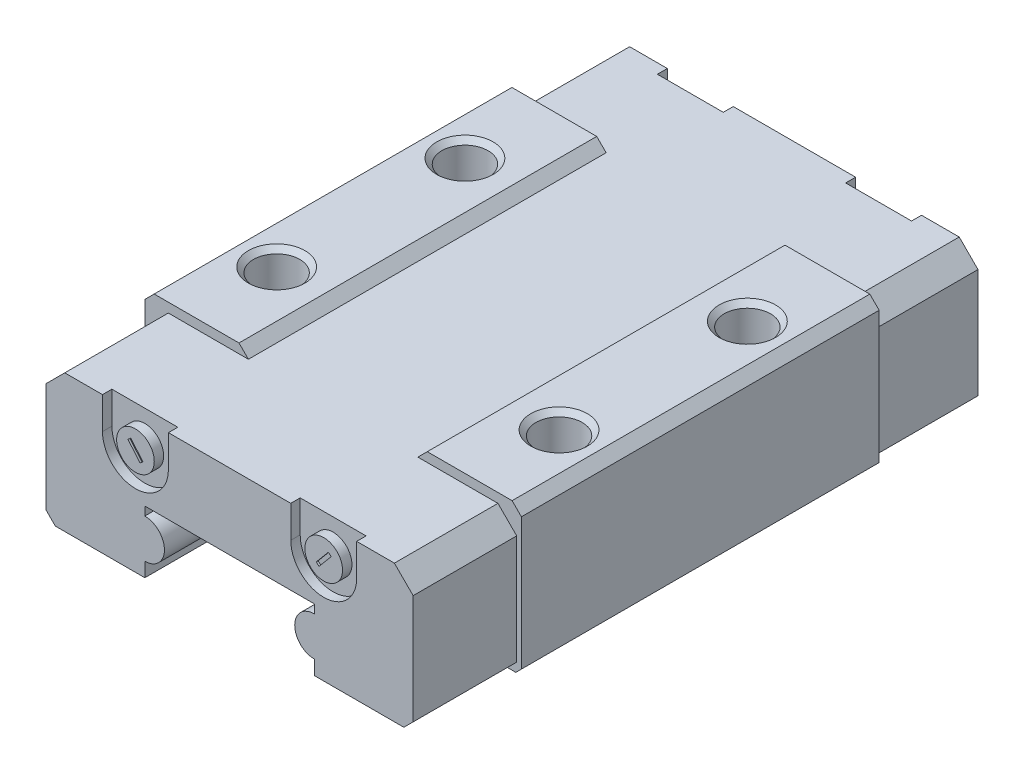
from build123d import *

# Parameters (mm, degrees)
BOSS_EXTRUDE1_DEPTH      = 9.5
BOSS_EXTRUDE1_DEPTH_BACK = 9.5
BOSS_EXTRUDE2_DEPTH      = 5.5
BOSS_EXTRUDE3_START      = -5.5
BOSS_EXTRUDE3_DEPTH      = 5.5
SKETCH4_R                = 1
CUT_EXTRUDE1_DEPTH       = 0.53
CUT_EXTRUDE2_START       = -0.5
SKETCH5_R                = 1
CUT_EXTRUDE2_DEPTH       = 0.5
LPATTERN1_COUNT          = 2
LPATTERN1_PITCH          = 10
LPATTERN1_COUNT_DIR2     = 2
LPATTERN1_PITCH_DIR2     = 15
CUT_EXTRUDE3_DEPTH       = 0.1
CUT_EXTRUDE4_DEPTH       = 0.1
CUT_EXTRUDE5_DEPTH       = 0.1
CUT_EXTRUDE6_DEPTH       = 0.1


with BuildPart() as part:
    # Sketch1 → Boss-Extrude1 (new, two sides: drawn at the far end of the back side and taken through both)
    with BuildSketch(Plane.XY.offset(-BOSS_EXTRUDE1_DEPTH_BACK)):
        with BuildLine():
            Line((-10, 7.305025253), (-10, 0.296984848))
            Line((-10, 0.296984848), (-9.703015152, 0))
            Line((-9.703015152, 0), (-4.5, 0))
            Line((-4.5, 0), (-4.5, 0.76))
            ThreePointArc((-4.5, 0.76), (-3.46, 1.8), (-4.5, 2.84))
            Line((-4.5, 2.84), (-4.5, 3.3))
            Line((-4.5, 3.3), (4.5, 3.3))
            Line((4.5, 3.3), (4.5, 2.84))
            ThreePointArc((4.5, 2.84), (3.46, 1.8), (4.5, 0.76))
            Line((4.5, 0.76), (4.5, 0))
            Line((4.5, 0), (9.703015152, 0))
            Line((9.703015152, 0), (10, 0.296984848))
            Line((10, 0.296984848), (10, 7.305025253))
            Line((10, 7.305025253), (9.505025253, 7.8))
            Line((9.505025253, 7.8), (5, 7.8))
            Line((5, 7.8), (4.5, 7.3))
            Line((4.5, 7.3), (-4.5, 7.3))
            Line((-4.5, 7.3), (-5, 7.8))
            Line((-5, 7.8), (-9.505025253, 7.8))
            Line((-9.505025253, 7.8), (-10, 7.305025253))
        make_face()
    extrude(amount=BOSS_EXTRUDE1_DEPTH + BOSS_EXTRUDE1_DEPTH_BACK)

    # Sketch2 → Boss-Extrude2 (add)
    with BuildSketch(Plane.XY.offset(9.5)):
        with BuildLine():
            Line((-9.75, 6.302979439), (-9.75, 0.494974747))
            Line((-9.75, 0.494974747), (-9.255025253, 0))
            Line((-9.255025253, 0), (-4.5, 0))
            Line((-4.5, 0), (-4.5, 0.76))
            ThreePointArc((-4.5, 0.76), (-3.46, 1.8), (-4.5, 2.84))
            Line((-4.5, 2.84), (-4.5, 3.3))
            Line((-4.5, 3.3), (4.5, 3.3))
            Line((4.5, 3.3), (4.5, 2.84))
            ThreePointArc((4.5, 2.84), (3.46, 1.8), (4.5, 0.76))
            Line((4.5, 0.76), (4.5, 0))
            Line((4.5, 0), (9.255025253, 0))
            Line((9.255025253, 0), (9.75, 0.494974747))
            Line((9.75, 0.494974747), (9.75, 6.302979439))
            Line((9.75, 6.302979439), (8.752979439, 7.3))
            Line((8.752979439, 7.3), (-8.752979439, 7.3))
            Line((-8.752979439, 7.3), (-9.75, 6.302979439))
        make_face()
    extrude(amount=BOSS_EXTRUDE2_DEPTH)

    # Sketch3 → Boss-Extrude3 (add)
    with BuildSketch(Plane.XY.offset(-9.5).offset(BOSS_EXTRUDE3_START)):
        with BuildLine():
            Line((-9.75, 6.302979439), (-9.75, 0.494974747))
            Line((-9.75, 0.494974747), (-9.255025253, 0))
            Line((-9.255025253, 0), (-4.5, 0))
            Line((-4.5, 0), (-4.5, 0.76))
            ThreePointArc((-4.5, 0.76), (-3.46, 1.8), (-4.5, 2.84))
            Line((-4.5, 2.84), (-4.5, 3.3))
            Line((-4.5, 3.3), (4.5, 3.3))
            Line((4.5, 3.3), (4.5, 2.84))
            ThreePointArc((4.5, 2.84), (3.46, 1.8), (4.5, 0.76))
            Line((4.5, 0.76), (4.5, 0))
            Line((4.5, 0), (9.255025253, 0))
            Line((9.255025253, 0), (9.75, 0.494974747))
            Line((9.75, 0.494974747), (9.75, 6.302979439))
            Line((9.75, 6.302979439), (8.752979439, 7.3))
            Line((8.752979439, 7.3), (-8.752979439, 7.3))
            Line((-8.752979439, 7.3), (-9.75, 6.302979439))
        make_face()
    extrude(amount=BOSS_EXTRUDE3_DEPTH)

    # Sketch4 → Cut-Extrude1 (cut)
    with BuildSketch(Plane.XY.offset(-15)):
        with BuildLine():
            Line((-6.75, 20), (-6.75, 5.6))
            ThreePointArc((-6.75, 5.6), (-5, 3.85), (-3.25, 5.6))
            Line((-3.25, 5.6), (-3.25, 18.82500207))
            Line((-3.25, 18.82500207), (3.25, 18.82500207))
            Line((3.25, 18.82500207), (3.25, 5.6))
            ThreePointArc((3.25, 5.6), (5, 3.85), (6.75, 5.6))
            Line((6.75, 5.6), (6.75, 20))
            Line((6.75, 20), (-6.75, 20))
        make_face()
        with Locations((5, 5.6)):
            Circle(SKETCH4_R, mode=Mode.SUBTRACT)
        with Locations((-5, 5.6)):
            Circle(SKETCH4_R, mode=Mode.SUBTRACT)
    extrude(amount=CUT_EXTRUDE1_DEPTH, mode=Mode.SUBTRACT)

    # Sketch5 → Cut-Extrude2 (cut)
    with BuildSketch(Plane.XY.offset(15).offset(CUT_EXTRUDE2_START)):
        with BuildLine():
            Line((-6.75, 20), (-6.75, 5.6))
            ThreePointArc((-6.75, 5.6), (-5, 3.85), (-3.25, 5.6))
            Line((-3.25, 5.6), (-3.25, 18.82500207))
            Line((-3.25, 18.82500207), (3.25, 18.82500207))
            Line((3.25, 18.82500207), (3.25, 5.6))
            ThreePointArc((3.25, 5.6), (5, 3.85), (6.75, 5.6))
            Line((6.75, 5.6), (6.75, 20))
            Line((6.75, 20), (-6.75, 20))
        make_face()
        with Locations((5, 5.6)):
            Circle(SKETCH5_R, mode=Mode.SUBTRACT)
        with Locations((-5, 5.6)):
            Circle(SKETCH5_R, mode=Mode.SUBTRACT)
    extrude(amount=CUT_EXTRUDE2_DEPTH, mode=Mode.SUBTRACT)

    # Sketch6 → Cut-Revolve1 (revolve, cut)
    with BuildSketch(Plane(origin=(7.5, 0, 0), x_dir=(0, 0, -1), z_dir=(1, 0, 0)), mode=Mode.PRIVATE) as cut_revolve1_sk:
        Polygon((-5, 7.8), (-3.5, 7.8), (-3.7705, 7.5295), (-3.7705, 4.009852156), (-5, 3.3), align=None)
    cut_revolve1 = revolve(cut_revolve1_sk.sketch.rotate(Axis((7.5, 3.3, 5), (0, 1, 0)), 180), axis=Axis((7.5, 3.3, 5), (0, 1, 0)), mode=Mode.SUBTRACT)

    # LPattern1: Cut-Revolve1 2 × 2
    with Locations(*[(-j * LPATTERN1_PITCH_DIR2, 0, -i * LPATTERN1_PITCH) for i in range(LPATTERN1_COUNT) for j in range(LPATTERN1_COUNT_DIR2) if (i, j) != (0, 0)]):
        add(cut_revolve1, mode=Mode.SUBTRACT)

    # Sketch8 → Cut-Extrude3 (cut)
    with BuildSketch(Plane.XY.offset(15)):
        Polygon((4.602001751, 5.281256539), (4.755210639, 5.152699017), (5.397998249, 5.918743461), (5.244789361, 6.047300983), align=None)
    extrude(amount=-CUT_EXTRUDE3_DEPTH, mode=Mode.SUBTRACT)

    # Sketch9 → Cut-Extrude4 (cut)
    with BuildSketch(Plane.XY.offset(15)):
        Polygon((-5.397998249, 5.918743461), (-4.755210639, 5.152699017), (-4.602001751, 5.281256539), (-5.244789361, 6.047300983), align=None)
    extrude(amount=-CUT_EXTRUDE4_DEPTH, mode=Mode.SUBTRACT)

    # Sketch10 → Cut-Extrude5 (cut)
    with BuildSketch(Plane.XY.offset(-15)):
        Polygon((4.602001751, 5.281256539), (4.755210639, 5.152699017), (5.397998249, 5.918743461), (5.244789361, 6.047300983), align=None)
    extrude(amount=CUT_EXTRUDE5_DEPTH, mode=Mode.SUBTRACT)

    # Sketch11 → Cut-Extrude6 (cut)
    with BuildSketch(Plane.XY.offset(-15)):
        Polygon((-5.397998249, 5.918743461), (-4.755210639, 5.152699017), (-4.602001751, 5.281256539), (-5.244789361, 6.047300983), align=None)
    extrude(amount=CUT_EXTRUDE6_DEPTH, mode=Mode.SUBTRACT)


solid = part.part
